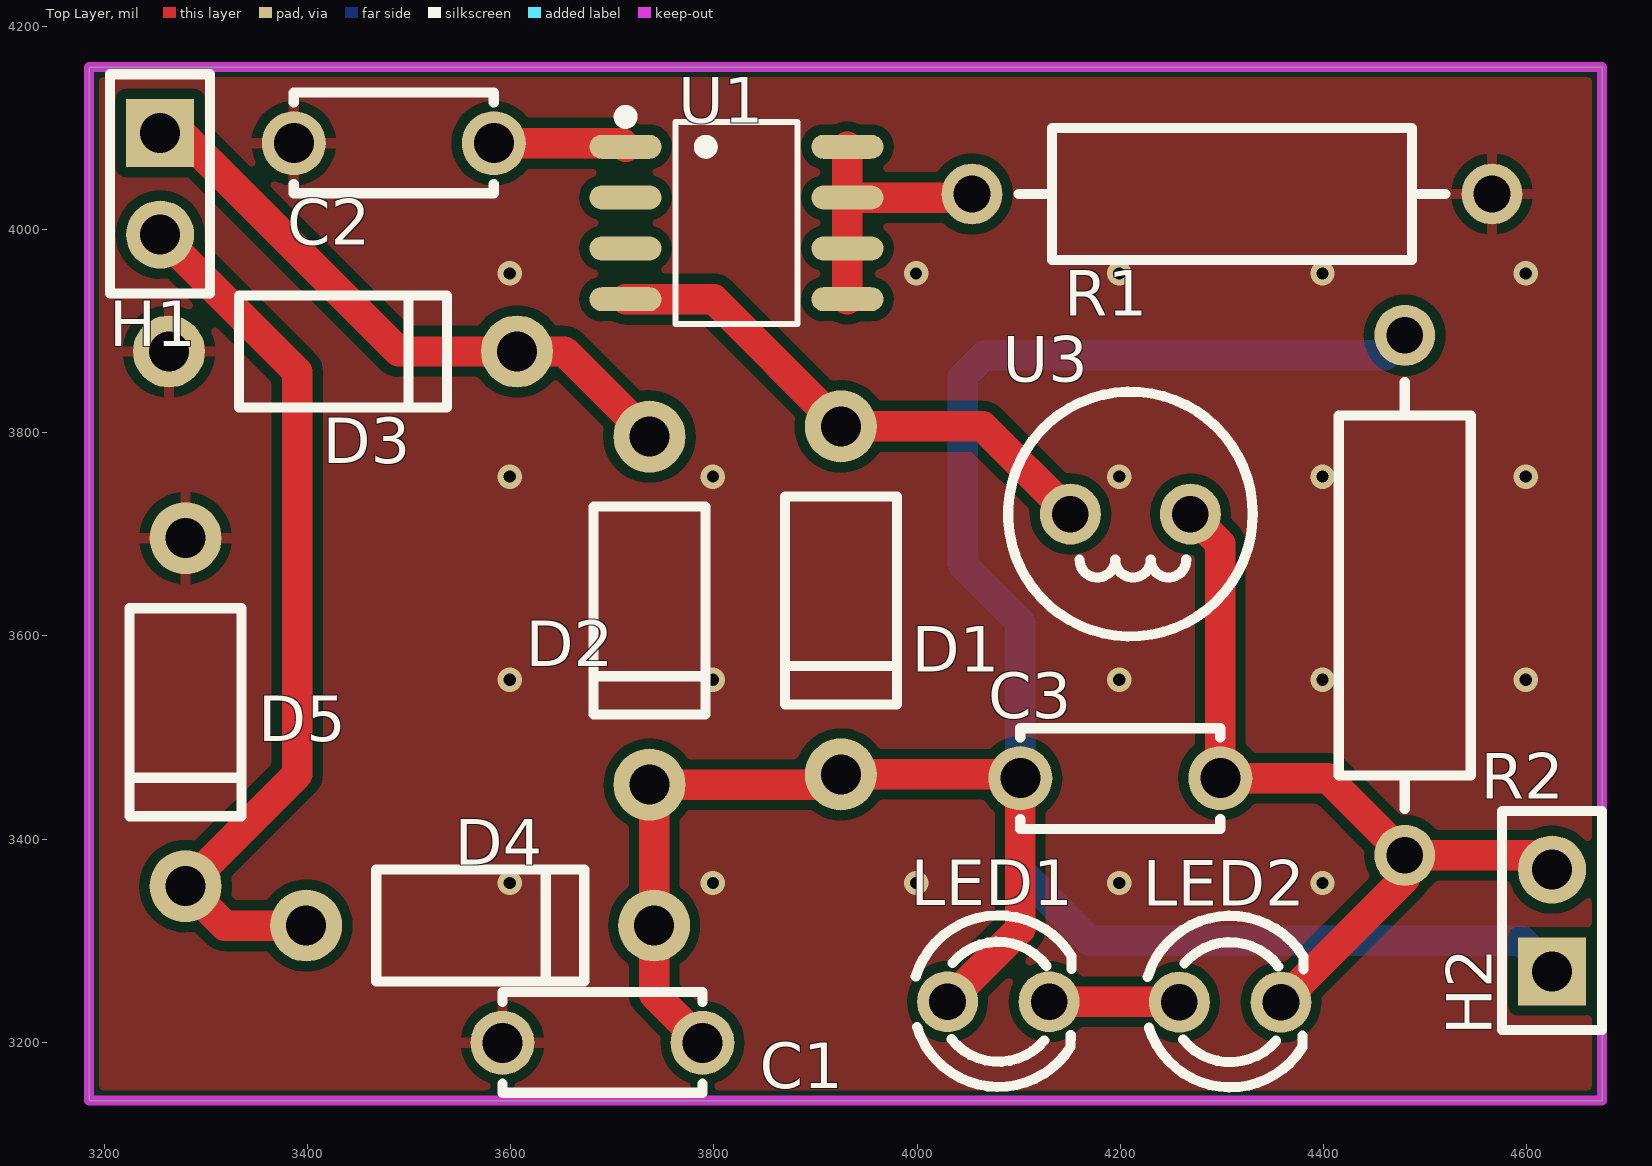
[diagram p0: Top Layer view]
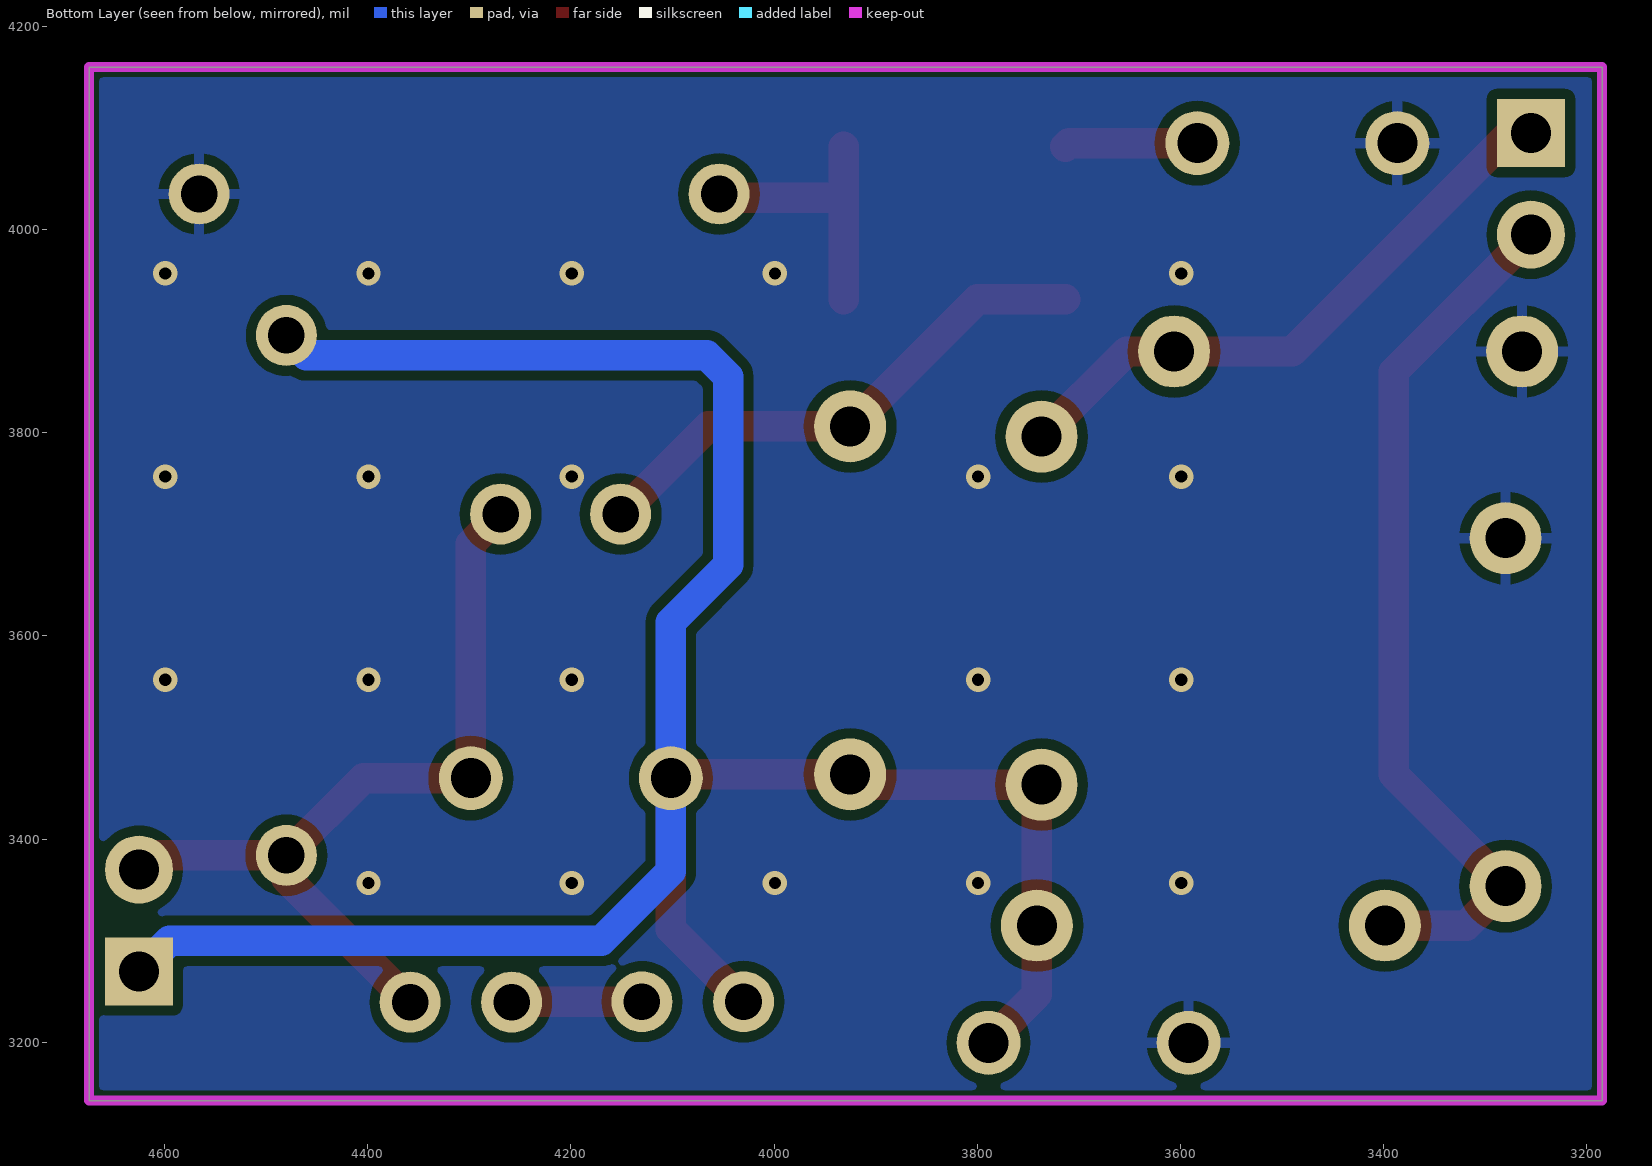
[diagram p1: Bottom Layer view, seen from below]
# Altium PCB MISC51823.pcbdoc
Units mil, origin at the board's own origin, x right, y up, seen from the top; angles counter-clockwise.
Board outline 1489.21 x 1017.24 mil, 2 copper layers (Top Layer, Bottom Layer), stack 62.206 mil thick; 16 components, 9 nets, 38 pads, 20 vias.

## Layer stack, top to bottom
Top Solder Mask Layer: solder mask 0.394, Dk 3.3
Top Layer: signal copper 1.379
Dielectric1: surface 59.449, FR4, Dk 4.5
Bottom Layer: signal copper 1.378
Bottom Solder Mask Layer: solder mask 0.394, Dk 3.3

## Board outline
3185,4160 3185,3142.76 4674.21,3142.76 4674.21,4160

## Design rules (kind name [scope] priority, off if disabled: settings)
BoardOutlineClearance copperThickness2oz_1 [All] p2 off: genericclearance=7.99 ignorepadtopadclearanceinfootprint=FALSE except(0: Arc-SplitContinuation Track-SplitContinuation SMDPad-SplitContinuation THPad-SplitContinuation Via-SplitContinuation Fill-SplitContinuation Region-SplitContinuation Poly-SplitContinuation Text-SplitContinuation Hole-SplitContinuation; 5.98: Arc-CutoutEdge SMDPad-CutoutEdge THPad-CutoutEdge Via-CutoutEdge Fill-CutoutEdge Region-CutoutEdge Text-CutoutEdge; 6.93: Hole-OutlineEdge Hole-CutoutEdge; 10: Poly-OutlineEdge Poly-CutoutEdge; 11.81: Arc-OutlineEdge Track-OutlineEdge SMDPad-OutlineEdge THPad-OutlineEdge Via-OutlineEdge Fill-OutlineEdge Region-OutlineEdge Text-OutlineEdge Track-CutoutEdge)
BoardOutlineClearance copperThickness1oz_1 [All] p4: genericclearance=4.02 ignorepadtopadclearanceinfootprint=FALSE except(0: Arc-SplitContinuation Track-SplitContinuation SMDPad-SplitContinuation THPad-SplitContinuation Via-SplitContinuation Fill-SplitContinuation Region-SplitContinuation Poly-SplitContinuation Text-SplitContinuation Hole-SplitContinuation; 6: SMDPad-CutoutEdge THPad-CutoutEdge Via-CutoutEdge Fill-CutoutEdge Region-CutoutEdge Text-CutoutEdge; 6.93: Hole-OutlineEdge Hole-CutoutEdge; 10: Poly-OutlineEdge Poly-CutoutEdge; 11.8: Arc-OutlineEdge Track-OutlineEdge SMDPad-OutlineEdge THPad-OutlineEdge Via-OutlineEdge Fill-OutlineEdge Region-OutlineEdge Text-OutlineEdge; 11.81: Arc-CutoutEdge Track-CutoutEdge)
Clearance copperThickness2oz [All] p1 off: gap=7.99 ignorepadtopadclearanceinfootprint=FALSE except(5.98: SMDPad-Track SMDPad-SMDPad THPad-Track SMDPad-THPad THPad-THPad Track-Via SMDPad-Via THPad-Via Via-Via Fill-Track Region-Track Fill-SMDPad Region-SMDPad Fill-THPad Region-THPad Fill-Via Region-Via Fill-Fill Fill-Region Region-Region Arc-Track Arc-SMDPad Arc-THPad Arc-Via Fill-Arc Region-Arc Arc-Arc Text-Track SMDPad-Text Text-THPad Text-Via Fill-Text Region-Text Arc-Text Text-Text; 6.93: Hole-Track Hole-SMDPad Hole-THPad Hole-Via Fill-Hole Region-Hole Hole-Arc Hole-Text; 10: Poly-Track Poly-SMDPad Poly-THPad Poly-Via Poly-Fill Poly-Region Poly-Poly Poly-Arc Poly-Text Poly-Hole)
Clearance copperThickness1oz [All] p3: gap=4.02 ignorepadtopadclearanceinfootprint=FALSE except(5.98: SMDPad-Track SMDPad-SMDPad THPad-Track SMDPad-THPad THPad-THPad Track-Via SMDPad-Via THPad-Via Via-Via Fill-Track Region-Track Fill-SMDPad Region-SMDPad Fill-THPad Region-THPad Fill-Via Region-Via Fill-Fill Fill-Region Region-Region; 6: Arc-Track Arc-SMDPad Arc-THPad Arc-Via Fill-Arc Region-Arc Arc-Arc Text-Track SMDPad-Text Text-THPad Text-Via Fill-Text Region-Text Arc-Text Text-Text; 6.93: Hole-Track Hole-SMDPad Hole-THPad Hole-Via Fill-Hole Region-Hole Hole-Arc Hole-Text; 10: Poly-Track Poly-SMDPad Poly-THPad Poly-Via Poly-Fill Poly-Region Poly-Poly Poly-Arc Poly-Text Poly-Hole)
DiffPairsRouting differentialPair [All] p1: maxlimit=6 minlimit=6 mostfreqgap=6 toplayer_minwidth=5 toplayer_prefwidth=10 toplayer_maxwidth=100 toplayer_mingap=6 toplayer_prefgap=6 toplayer_maxgap=6 bottomlayer_minwidth=5 bottomlayer_prefwidth=10 bottomlayer_maxwidth=100 bottomlayer_mingap=6 bottomlayer_prefgap=6 bottomlayer_maxgap=6 maxuncoupledlength=10
HoleToHoleClearance otherClearance [All] p1: gap=11.81 allowstackedmicrovias=TRUE
Length netLength [All] p1: minlimit=0 maxlimit=0
MatchedLengths netLengthTolerance [All] p1: tolerance=1000
PasteMaskExpansion pasteMaskExpansion [All] p1: expansion=0
PlaneConnect innerPlane [All] p1: planeconnectstyle=Relief reliefexpansion=20 reliefentries=4 reliefconductorwidth=10 reliefairgap=10
PolygonConnect copperRegion [(InNet('GND'))] p1: connectstyle=Relief reliefconductorwidth=10 reliefentries=4 polygonreliefangle="90 Angle" airgapwidth=10 via.connectstyle=Relief via.reliefconductorwidth=10 via.reliefentries=4 via.polygonreliefangle="90 Angle" via.airgapwidth=10
RoutingVias viaSize [All] p1: holewidth=12.01 width=24.02 viastyle="Through Hole" minholewidth=11.81 minwidth=19.68 maxholewidth=248.03 maxwidth=393.7
SolderMaskExpansion solderMaskExpansion [IsVia] p1: expansion=-1000 istentingtop=TRUE
SolderMaskExpansion solderMaskExpansion [All] p2: expansion=2 istentingtop=FALSE
Width copperThickness2oz_2 [All] p1 off: maxlimit=100 minlimit=8 preferedwidth=10
Width copperThickness1oz_2 [All] p2: maxlimit=100 minlimit=5 preferedwidth=10

## Components (designator, comment, footprint, x,y, rotation, side; value= is the part's Value field where it differs from the comment)
C1 "100nF" CAP-TH_L5.0-W2.5-P5.00-D1.0 3690.39,3199.61 r180 top
C2 "100nF" CAP-TH_L5.0-W2.5-P5.00-D1.0 3485,4085 r180 top
C3 "100nF" CAP-TH_L5.0-W2.5-P5.00-D1.0 4200,3460 r0 top
D1 "" DO_1N4007 3925,3635 r90 top
D2 "" DO_1N4007 3736.68,3625 r90 top
D3 "" DO_1N4007 3435,3880 r180 top
D4 "" DO_1N4007 3570,3315 r180 top
D5 "" DO_1N4007 3280,3525 r90 top
H1 "" HDR-TH_2P-P2.54-V-F 3255,4045 r270 top
H2 "" HDR-TH_2P-P2.54-V-F 4625,3320 r90 top
LED1 "" LED_TH-3mm 4080,3240 r0 top
LED2 "" LED_TH-3mm 4308.2,3239.58 r0 top
R1 "10kΩ" Res_1/2W 4310,4035 r0 top
R2 "10kΩ" Res_1/2W 4480,3640 r90 top
U1 "PT4501C" SOP-8_L4.9-W3.9-P1.27-LS6.0-BL-EP 3822.31,4006.5 r270 top
U3 "L6_8MM" IND-TH_BD6.00-P3.00-D0.6 4210,3720 r0 top

## Footprints (in the part's own frame and the unit in brackets; to place one, negate y for a bottom-side part, rotate by r counter-clockwise, add the part's x,y. Pads: shape width x height; smd on the part's side, far side on the other; paste and mask are expansions set on the pad)
CAP-TH_L5.0-W2.5-P5.00-D1.0 [mm]
  round 1.6 hole 1: 1(-2.5,0) 2(2.5,0)
  silkscreen extent -2.5,-1.27 2.5,1.25
DO_1N4007 [mm]
  round 1.8 hole 1 paste+0 mask+0.051: 1(-4.35,0) 2(4.35,0)
  silkscreen extent -2.6,-1.4 2.6,1.4
HDR-TH_2P-P2.54-V-F [mm]
  rect 1.7x1.7 hole 1: 1(-1.27,0)
  round 1.7 hole 1: 2(1.27,0)
  silkscreen extent -2.74,-1.25 2.74,1.25
IND-TH_BD6.00-P3.00-D0.6 [mil]
  round 60 hole 36 paste+0 mask+1.97: 1(-59.06,0) 2(59.05,0)
  silkscreen extent -120,-120 120,120
LED_TH-3mm [mil]
  round 60 hole 36 paste+0 mask+2: 1(-50,0) 2(50,0)
  silkscreen extent -81,-84 72,85
Res_1/2W [mil]
  round 60 hole 36 paste+0 mask+2: 1(-255.91,0) 2(255.9,0)
  silkscreen extent -210,-65 210,65
SOP-8_L4.9-W3.9-P1.27-LS6.0-BL-EP [mm]
  oval 0.6x1.8 smd: 1(-1.905,-2.772) 2(-0.635,-2.772) 3(0.635,-2.772) 4(1.905,-2.772) 5(1.905,2.772) 6(0.635,2.772) 7(-0.635,2.772) 8(-1.905,2.772)
  silkscreen extent -2.8,-2.92 2.53,1.52

## Via types
v1: diameter 24.02, hole 12, Top Layer to Bottom Layer, 20 vias

## Nets (pads, with @x,y where several pads share a name; then routed paths per layer and width w, separated by ;. In a path a pad name is that pad's centre, name@x,y a point inside that pad or via, vN(x,y) a via of type N, cw(c..) or ccw(c..) an arc to the next point about the centre after c; other vN are vias at no path point)
$1N3: R1.1 U1.5 U1.6 U1.7 U1.8 | length 274.1
  Top Layer w30: U1.5 U1.6 U1.7 ; U1.8 U1.7 ; R1.1 4050.59,4031.5 U1.7
$1N5: D1.2 U1.4 U3.1 | length 525.4
  Top Layer w30: U1.4 3799.76,3931.5 D1.2 4064.68,3806.26 U3.1
$1N6: C3.2 H2.2 LED2.2 R2.1 U3.2 | length 831
  Top Layer w30: U3.2@4269.06,3720 4298.43,3690.63 C3.2 4404.1,3460 R2.1 ; LED2.2 4480,3361.38 R2.1 ; H2.2 4610.9,3384.09 R2.1
$1N8: LED1.2 LED2.1 | length 128.4
  Top Layer w30: LED1.2 4257.78,3240 LED2.1
$1N12: D4.2 D5.1 H1.2 | length 877.5
  Top Layer w30: H1.2 3390,3860 3390,3463.74 D5.1 3318.74,3315 D4.2
$1N13: D2.2 D3.1 H1.1 | length 605.4
  Top Layer w30: H1.1 3275,4095 3490,3880 D3.1 3652.94,3880 D2.2
$1N16: C1.1 C3.1 D1.1 D2.1 D4.1 H2.1 LED1.1 R2.2 | length 2422.1
  Top Layer w30: C1.1 3741.26,3247.16 D4.1 3741.26,3449.16 D2.1 3915,3453.74 D1.1 4097.84,3463.74 C3.1 4101.57,3311.57 LED1.1
  Bottom Layer w30: R2.2 4460.31,3876.21 4066.21,3876.21 4045,3855 4045,3670 4101.57,3613.43 C3.1 4101.57,3368.43 4170,3300 4595,3300 H2.1
GND: C1.2 C2.2 D3.2 D5.2 R1.2
  other v1: 3599.1,3356.86 3799.1,3356.86 3999.1,3356.86 4199.1,3356.86 4399.1,3356.86 3599.1,3556.86 3799.1,3556.86 4199.1,3556.86 4399.1,3556.86 4599.1,3556.86 3599.1,3756.86 3799.1,3756.86 4199.1,3756.86 4399.1,3756.86 4599.1,3756.86 3599.1,3956.86 3999.1,3956.86 4199.1,3956.86 4399.1,3956.86 4599.1,3956.86
VDD: C2.1 U1.1 | length 131.2
  Top Layer w30: C2.1 3709.66,4085 U1.1
pads on no net: U1.2 U1.3

## Polygon pours and split planes (outlines as drawn)
GND on Bottom Layer (solid, remove dead copper, pour order 2): 3085,4330 3085,3065 4785,3065 4785,4330
GND on Top Layer (solid, remove dead copper, pour order 0): 3000,4325 3000,3000 4840,3000 4840,4325

## Keep-outs
Board Outline Layer:
  the board outline again, w10